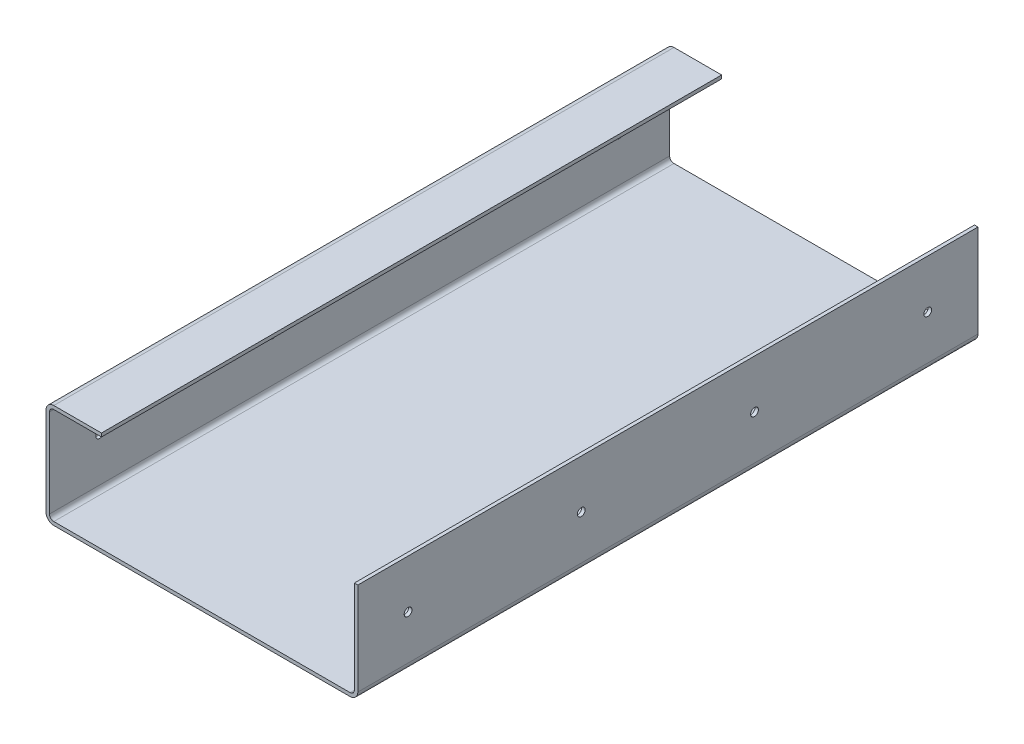
from build123d import *

# Parameters (mm, degrees)
BOSS_EXTRUDE1_DEPTH = 716
SKETCH2_R           = 4.5
CUT_EXTRUDE1_DEPTH  = 716


with BuildPart() as part:
    # Sketch1 → Boss-Extrude1 (new body)
    with BuildSketch(Plane.XY):
        with BuildLine():
            Line((0, 0), (-55, 0))
            ThreePointArc((-55, 0), (-61.363961031, -2.636038969), (-64, -9))
            Line((-64, -9), (-64, -111))
            ThreePointArc((-64, -111), (-61.363961031, -117.363961031), (-55, -120))
            Line((-55, -120), (287, -120))
            ThreePointArc((287, -120), (293.363961031, -117.363961031), (296, -111))
            Line((296, -111), (296, -4))
            Line((296, -4), (292, -4))
            Line((292, -4), (292, -111))
            ThreePointArc((292, -111), (290.535533906, -114.535533906), (287, -116))
            Line((287, -116), (-55, -116))
            ThreePointArc((-55, -116), (-58.535533906, -114.535533906), (-60, -111))
            Line((-60, -111), (-60, -9))
            ThreePointArc((-60, -9), (-58.535533906, -5.464466094), (-55, -4))
            Line((-55, -4), (0, -4))
            Line((0, -4), (0, 0))
        make_face()
    extrude(amount=BOSS_EXTRUDE1_DEPTH)

    # Sketch2 → Cut-Extrude1 (cut)
    with BuildSketch(Plane.ZY.offset(64)):
        with Locations(Location((58, -60, 0), (0, 0, 270))):
            Circle(SKETCH2_R)
        with Locations(Location((258, -60, 0), (0, 0, 270))):
            Circle(SKETCH2_R)
        with Locations(Location((458, -60, 0), (0, 0, 270))):
            Circle(SKETCH2_R)
        with Locations(Location((658, -60, 0), (0, 0, 270))):
            Circle(SKETCH2_R)
    extrude(amount=-CUT_EXTRUDE1_DEPTH, mode=Mode.SUBTRACT)


solid = part.part
